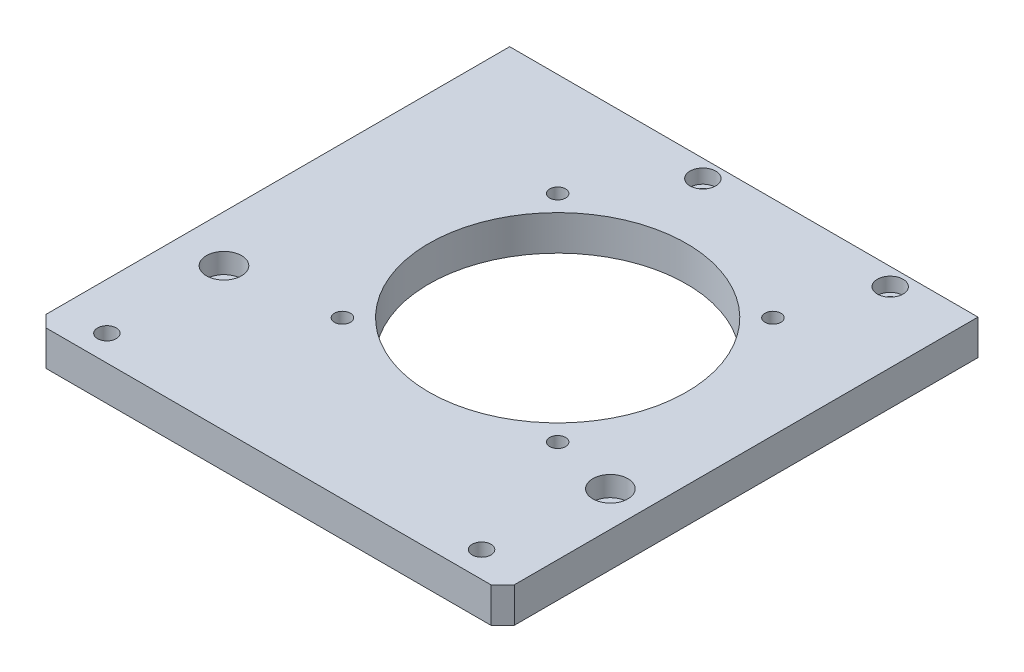
SolidWorks part; units mm, degrees
ref_plane "Front Plane" through (0, 0, 0) normal (0, 0, 1) x (1, 0, 0)
ref_plane "Top Plane" through (0, 0, 0) normal (0, 1, 0) x (1, 0, 0)
ref_plane "Right Plane" through (0, 0, 0) normal (1, 0, 0) x (0, 0, -1)
sketch "Sketch1" plane through (0, 0, 0) normal (0, 1, 0) x (1, 0, 0)
  line L1 (100, 91.5) -> (-100, 91.5)
  line L2 (100, 91.5) -> (100, -91.5)
  line L3 (100, -91.5) -> (-100, -91.5)
  line L4 (-100, 91.5) -> (-100, -91.5)
  line L5 (100, 91.5) -> (-100, -91.5) construction
  line L6 (100, -91.5) -> (-100, 91.5) construction
  point P0 (0, 0)
  dimension "D1" = 200
  dimension "D2" = 183
extrude "Boss-Extrude1" add sketch "Sketch1" along normal blind 15
hole_wizard "M8 Tapped Hole1" positions "Sketch4" profile "Sketch3" tap size "M8" standard "Iso" end condition through all
sketch "Sketch4" plane through (0, 15, 0) normal (0, 1, 0) x (-1, 0, 0)
  point P0 (35.4619, -62.4619)
  point P1 (-56.4619, -62.4619)
  point P3 (35.4619, 29.4619)
  point P5 (-56.4619, 29.4619)
sketch "Sketch3" plane through (-35.4619, 15, -62.4619) normal (1, 0, 0) x (0, 0, 1)
  line L0 (0, 0) -> (0, 15)
  line L1 (0, 15) -> (3.4, 15)
  line L2 (3.4, 15) -> (3.4, 0)
  line L5 (3.4, 0) -> (0, 0)
  line L11 (0, -6.35) -> (0, 107.95) construction
  dimension "通孔螺纹孔钻头直径" = 6.8
  dimension "通孔螺纹孔钻头深度" = 15
cosmetic thread "Cosmetic Thread1" parameters "D2"=8
cosmetic thread "Cosmetic Thread2" parameters "D2"=8
cosmetic thread "Cosmetic Thread3" parameters "D2"=8
cosmetic thread "Cosmetic Thread4" parameters "D2"=8
sketch "Sketch11" plane through (0, 0, -91.5) normal (0, 0, -1) x (-1, 0, 0)
  line L1 (-100, 15) -> (100, 15)
  line L2 (-100, 15) -> (-100, 0)
  line L3 (-100, 0) -> (100, 0)
  line L4 (100, 15) -> (100, 0)
extrude "Boss-Extrude3" add sketch "Sketch11" along normal blind 15
hole_wizard "CBORE for M6 Hex Socket Head Cap Screw1" positions "Sketch6" profile "Sketch5" counterbore size "M6" standard "ISO" end condition through all
sketch "Sketch6" plane through (0, 15, 0) normal (0, 1, 0) x (-1, 0, 0)
  line L0 (-100, 91.5) -> (-100, -106.5) construction
  line L2 (100, -106.5) -> (-100, -106.5) construction
  point P0 (-70, -99)
  point P1 (10, -99)
  dimension "D1" = 30
  dimension "D2" = 80
  dimension "D3" = 7.5
  dimension "D4" = 7.5
sketch "Sketch5" plane through (70, 15, -99) normal (1, 0, 0) x (0, 0, 1)
  line L0 (0, 0) -> (0, 15)
  line L1 (0, 15) -> (3.3, 15)
  line L3 (3.3, 15) -> (3.3, 6)
  line L4 (3.3, 6) -> (5.5, 6)
  line L5 (5.5, 6) -> (5.5, 0)
  line L7 (5.5, 0) -> (0, 0)
  line L11 (0, -6.35) -> (0, 107.95) construction
  dimension "通孔孔直径" = 6.6
  dimension "通孔孔深度" = 15
  dimension "柱形沉头孔直径" = 11
  dimension "柱形沉头孔深度" = 6
hole_wizard "CBORE for M8 Hex Socket Head Cap Screw1" positions "Sketch8" profile "Sketch7" counterbore size "M8" standard "Iso" end condition through all
sketch "Sketch8" plane through (0, 15, 0) normal (0, 1, 0) x (-1, 0, 0)
  line L8 (-75.0457, 507) -> (-75.0457, 506.5) construction
  line L9 (-100, 507) -> (1500, 507) construction
  line L10 (1500, 506.5) -> (-100, 506.5) construction
  line L13 (-75.0457, 506.75) -> (-72.5016, 506.75) construction
  line L17 (100, -106.5) -> (-100, -106.5) construction
  line L18 (0, 0) -> (0, -91.8336) construction
  point P0 (-85, 35.5)
  point P241 (80, 35.5)
  dimension "D1" = 142
  dimension "D2" = 165
  dimension "D3" = 15
sketch "Sketch7" plane through (85, 15, 35.5) normal (1, 0, 0) x (0, 0, 1)
  line L0 (0, 0) -> (0, 15)
  line L1 (0, 15) -> (4.5, 15)
  line L3 (4.5, 15) -> (4.5, 8.6)
  line L4 (4.5, 8.6) -> (7.5, 8.6)
  line L5 (7.5, 8.6) -> (7.5, 0)
  line L7 (7.5, 0) -> (0, 0)
  line L11 (0, -6.35) -> (0, 107.95) construction
  dimension "通孔孔直径" = 9
  dimension "通孔孔深度" = 15
  dimension "柱形沉头孔直径" = 15
  dimension "柱形沉头孔深度" = 8.6
sketch "Sketch9" plane through (0, 0, 91.5) normal (0, 0, 1) x (1, 0, 0)
  line L1 (-100, 15) -> (100, 15)
  line L2 (-100, 15) -> (-100, 0)
  line L3 (-100, 0) -> (100, 0)
  line L4 (100, 15) -> (100, 0)
extrude "Boss-Extrude2" add sketch "Sketch9" along normal blind 5
sketch "Sketch10" plane through (0, 15, 0) normal (0, 1, 0) x (1, 0, 0)
  line L0 (100, -96.5) -> (-100, -96.5) construction
  line L1 (-100, 106.5) -> (-100, -96.5) construction
  line L2 (100, -96.5) -> (100, 106.5) construction
  circle A0 centre (-80, -85.5) radius 4
  circle A1 centre (80, -85.5) radius 4
  dimension "D5" = 8
  dimension "D6" = 8
  dimension "D1" = 11
  dimension "D2" = 11
  dimension "D3" = 20
  dimension "D4" = 20
extrude "Cut-Extrude2" cut sketch "Sketch10" against normal through all
chamfer "Chamfer1" distance 5 angle 45 2 edges at (-100, 7.5, 96.5) (100, 7.5, 96.5)
sketch "Sketch12" plane through (0, 15, 0) normal (0, 1, 0) x (1, 0, 0)
  circle A0 centre (10.5, 16.5) radius 55
  dimension "D1" = 110
extrude "Cut-Extrude3" cut sketch "Sketch12" against normal through all
